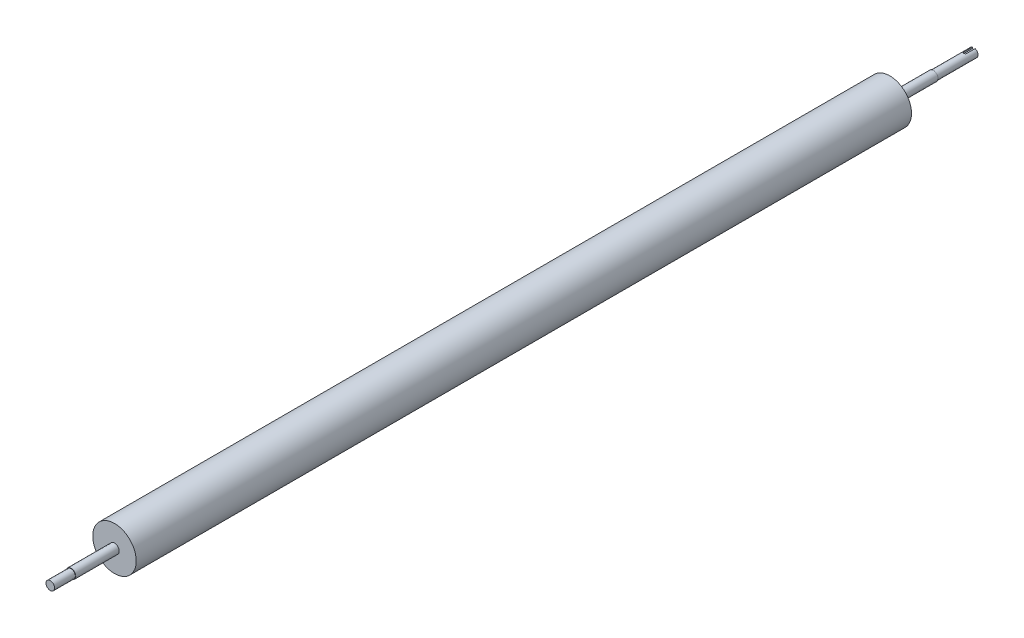
SolidWorks part; units mm, degrees
material "1060 合金"
ref_plane "前视基准面" through (0, 0, 0) normal (0, 0, 1) x (1, 0, 0)
ref_plane "上视基准面" through (0, 0, 0) normal (0, 1, 0) x (1, 0, 0)
ref_plane "右视基准面" through (0, 0, 0) normal (1, 0, 0) x (0, 0, -1)
sketch "草图1" plane through (0, 0, 0) normal (0, 0, 1) x (1, 0, 0)
  circle A0 centre (0, 0) radius 38
  dimension "D1" = 76
extrude "凸台-拉伸1" add sketch "草图1" along normal mid plane 1356
sketch "草图2" plane through (0, 0, 678) normal (0, 0, 1) x (1, 0, 0)
  circle A0 centre (0, 0) radius 7.5
  dimension "D1" = 15
extrude "凸台-拉伸2" add sketch "草图2" along normal mid plane 293.5
mirror "镜向1" about plane through (0, 0, 0) normal (0, 0, 1) of "凸台-拉伸2"
sketch "草图3" plane through (0, 0, 678) normal (0, 0, 1) x (1, 0, 0)
  circle A0 centre (0, 0) radius 8.25
  dimension "D1" = 16.5
extrude "凸台-拉伸4" add sketch "草图3" along normal blind 76 contours A0
sketch "草图4" plane through (0, 0, -678) normal (0, 0, -1) x (-1, 0, 0)
  circle A0 centre (0, 0) radius 8.25
  dimension "D1" = 16.5
extrude "凸台-拉伸5" add sketch "草图4" along normal blind 76
sketch "草图6" plane through (0, 0, 0) normal (0, 1, 0) x (1, 0, 0)
  line L0 (0, -824.75) -> (0, -809.75) construction
  line L3 (-7.5, -824.75) -> (7.5, -824.75) construction
  line L4 (-2.5, -824.75) -> (-2.5, -809.75)
  line L5 (2.5, -824.75) -> (2.5, -809.75)
  arc A2 (-2.5, -824.75) -> (2.5, -824.75) centre (0, -824.75) ccw
  arc A3 (2.5, -809.75) -> (-2.5, -809.75) centre (0, -809.75) ccw
  point P5 (0, -817.25)
  dimension "D1" = 5
  dimension "D2" = 15
extrude "切除-拉伸2" cut sketch "草图6" against normal blind 3 from offset 7.5
mirror "镜向2" about plane through (0, 0, 0) normal (0, 0, 1) of "切除-拉伸2"
ref_plane "基准面1" through (-2.5, 7.0711, -824.75) normal (-0.9428, -0.3333, 0) x (0, 0, 1)
sketch "草图9" plane through (0, 0, 824.75) normal (0, 0, 1) x (1, 0, 0)
  circle A0 centre (0, 0) radius 14.9961
extrude "切除-拉伸4" cut sketch "草图9" against normal blind 34.45
